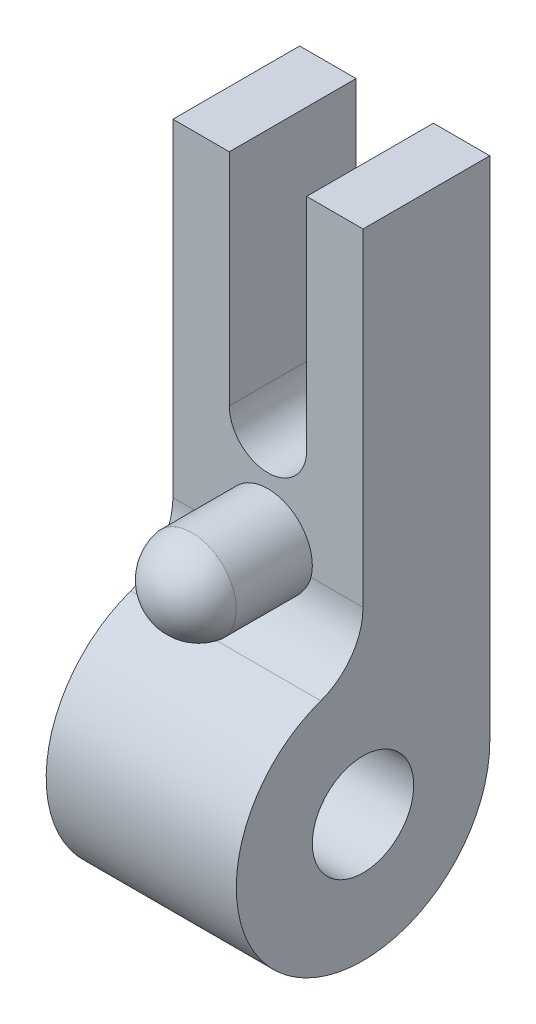
from build123d import *

# Parameters (mm, degrees)
SKETCH1_W           = 15
SKETCH1_H           = 20
BOSS_EXTRUDE1_DEPTH = 50
FILLET1_RADIUS      = 10
FILLET1_LENGTH      = 15
SKETCH2_R           = 4
CUT_EXTRUDE1_DEPTH  = 54.150729064
CUT_EXTRUDE2_DEPTH  = 54.150729064
FILLET2_R           = 5
SKETCH4_R           = 3.5
BOSS_EXTRUDE2_DEPTH = 6
DOME1_FACE_RADIUS   = 3.5
DOME1_HEIGHT        = 3
CUT_EXTRUDE3_DEPTH  = 55.371407941


with BuildPart() as part:
    # Sketch1 → Boss-Extrude1 (new body)
    with BuildSketch(Plane(origin=(0, 0, 0), x_dir=(1, 0, 0), z_dir=(0, 1, 0))):
        Rectangle(SKETCH1_W, SKETCH1_H)
    extrude(amount=BOSS_EXTRUDE1_DEPTH)

    # Fillet1: full round fillet: the end face becomes a half cylinder, R = half its width
    fillet1_face = Plane((0, 0, 0), x_dir=(-1, 0, 0), z_dir=(0, -1, 0))  # on the end face: x along it, z out of the body
    fillet1_slab = fillet1_face.offset(-FILLET1_RADIUS / 2) * Box(FILLET1_LENGTH, 2 * FILLET1_RADIUS, FILLET1_RADIUS, mode=Mode.PRIVATE)  # the body's end, R deep
    fillet1_round = Plane((0, 10, 0), x_dir=(0, -1, 0), z_dir=(-1, 0, 0)) * Cylinder(FILLET1_RADIUS, FILLET1_LENGTH, mode=Mode.PRIVATE)  # its axis R under the face
    add(fillet1_slab - fillet1_round, mode=Mode.SUBTRACT)

    # Sketch2 → Cut-Extrude1 (cut, through all)
    with BuildSketch(Plane.ZY.offset(7.5)):
        with Locations((0, 10)):
            Circle(SKETCH2_R)
    extrude(amount=-CUT_EXTRUDE1_DEPTH, mode=Mode.SUBTRACT)

    # Sketch3 → Cut-Extrude2 (cut, through all)
    with BuildSketch(Plane.ZY.offset(7.5)):
        with BuildLine():
            Line((0, 20), (0, 50))
            Line((0, 50), (10, 50))
            Line((10, 50), (10, 10))
            ThreePointArc((10, 10), (7.071067812, 17.071067812), (0, 20))
        make_face()
    extrude(amount=-CUT_EXTRUDE2_DEPTH, mode=Mode.SUBTRACT)

    # Fillet2
    fillet2_edges = [part.edges().sort_by_distance(p)[0] for p in [
        (0, 20, 0),
    ]]
    fillet(fillet2_edges, radius=FILLET2_R)

    # Sketch4 → Boss-Extrude2 (add)
    with BuildSketch(Plane.XY):
        with Locations(Location((0, 25, 0), (0, 0, 194.18798624))):
            Circle(SKETCH4_R)
    extrude(amount=BOSS_EXTRUDE2_DEPTH)

    # Dome1: a dome of height H over a round flat face of radius A is a cap of a sphere of radius (A * A + H * H) / (2 * H)
    dome1_r = (DOME1_FACE_RADIUS * DOME1_FACE_RADIUS + DOME1_HEIGHT * DOME1_HEIGHT) / (2 * DOME1_HEIGHT)
    dome1_base = Plane((0, 25, 6), z_dir=(0, 0, 1))
    with Locations(dome1_base.offset(DOME1_HEIGHT - dome1_r)):
        dome1_ball = Sphere(dome1_r, mode=Mode.PRIVATE)
    add(split(dome1_ball, bisect_by=dome1_base, keep=Keep.TOP, mode=Mode.PRIVATE))

    # Sketch5 → Cut-Extrude3 (cut, through all)
    with BuildSketch(Plane(origin=(0, 0, -10), x_dir=(-1, 0, 0), z_dir=(0, 0, -1))):
        with BuildLine():
            Line((3.05, 50), (3.05, 32.634868852))
            ThreePointArc((3.05, 32.634868852), (0, 29.584868852), (-3.05, 32.634868852))
            Line((-3.05, 32.634868852), (-3.05, 50))
            ThreePointArc((-3.05, 50), (0, 53.05), (3.05, 50))
        make_face()
    extrude(amount=-CUT_EXTRUDE3_DEPTH, mode=Mode.SUBTRACT)


solid = part.part
